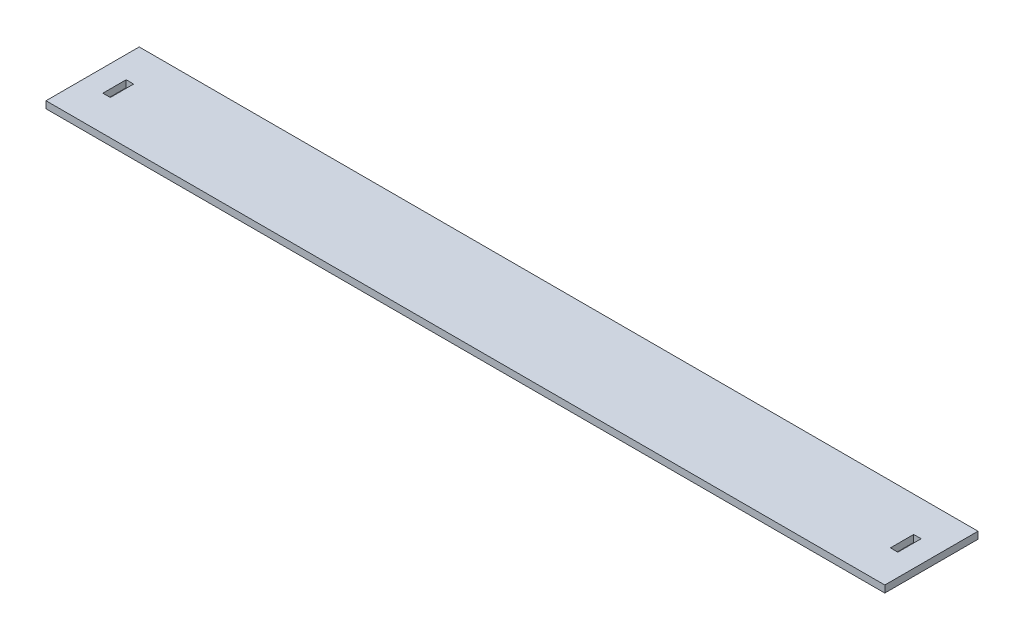
from build123d import *

# Parameters (mm, degrees)
SKETCH1_W           = 360
SKETCH1_H           = 40
BOSS_EXTRUDE1_DEPTH = 3
SKETCH2_W           = 3.2
SKETCH2_H           = 10
CUT_EXTRUDE1_DEPTH  = 10


with BuildPart() as part:
    # Sketch1 → Boss-Extrude1 (new body)
    with BuildSketch(Plane(origin=(0, 0, 0), x_dir=(1, 0, 0), z_dir=(0, 1, 0))):
        Rectangle(SKETCH1_W, SKETCH1_H)
    extrude(amount=BOSS_EXTRUDE1_DEPTH)

    # Sketch2 → Cut-Extrude1 (cut)
    with BuildSketch(Plane(origin=(0, 3, 0), x_dir=(1, 0, 0), z_dir=(0, 1, 0))):
        with Locations((-169, 0)):
            Rectangle(SKETCH2_W, SKETCH2_H)
        with Locations((169, 0)):
            Rectangle(SKETCH2_W, SKETCH2_H)
    extrude(amount=-CUT_EXTRUDE1_DEPTH, mode=Mode.SUBTRACT)


solid = part.part
